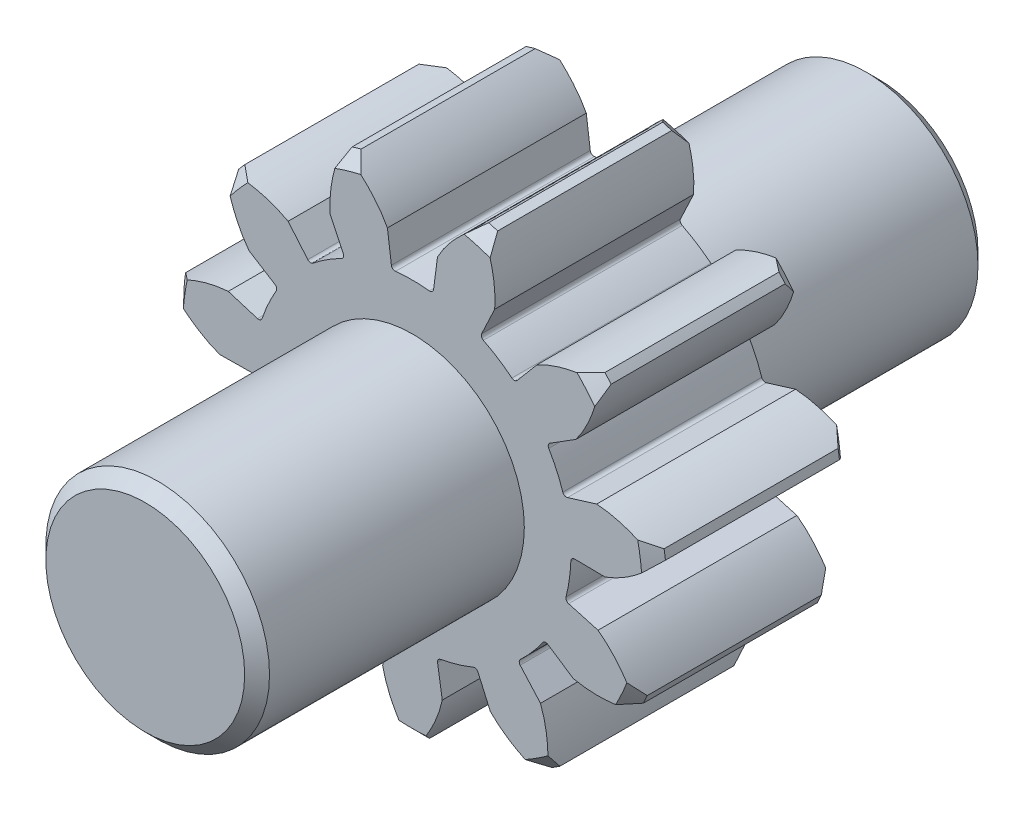
SolidWorks part; units mm, degrees
ref_plane "Middle plane" through (0, 0, 0) normal (0, 0, 1) x (1, 0, 0)
ref_plane "Top Plane" through (0, 0, 0) normal (0, 1, 0) x (1, 0, 0)
ref_plane "Right Plane" through (0, 0, 0) normal (1, 0, 0) x (0, 0, -1)
sketch "Spur gear" plane through (0, 0, 0) normal (0, 0, 1) x (1, 0, 0)
  line L0 (0, 0) -> (-2.3482, 16.3321) construction
  line L2 (-2.0154, 15.3734) -> (0, 0)
  line L3 (0, 0) -> (0, 52) construction
  line L4 (2.3482, 16.3321) -> (0, 0) construction
  line L6 (0, 0) -> (2.0154, 15.3734)
  circle A0 centre (0, 0) radius 15.5049
  circle A1 centre (0, 0) radius 12.75
  arc A2 (2.3482, 16.3321) -> (-2.3482, 16.3321) centre (0, 0) ccw
  circle A3 centre (0, 0) radius 19.5
  spline S0 degree 4 poles (0.7936, 14.8906) (0.7924, 14.9201) (0.7881, 14.9788) (0.7725, 15.0958) (0.7289, 15.316) (0.6484, 15.6067) (0.4539, 16.1447) (0.0492, 16.9597) (-0.6377, 17.9757) (-1.7913, 19.243) (-3.3499, 20.5096) (-5.2443, 21.6406) (-7.4338, 22.5657) (-9.7197, 23.2127) (-12.0632, 23.5974) (-14.5507, 23.7418) (-17.633, 23.5986) (-21.2621, 22.9576) (-25.3266, 21.6048) (-29.5547, 19.4226) (-33.4233, 16.6565) (-36.4497, 13.8025) (-38.7654, 11.0977) (-40.5023, 8.6952) (-41.7738, 6.6932) (-43.2134, 4.102) (-44.4514, 1.4058) (-45.4859, -1.3736) (-46.4831, -4.7889) (-47.0485, -7.396) (-47.4104, -9.7431) (-47.6077, -11.655) (-47.6802, -12.5487) (-47.7381, -13.4181) (-47.7759, -14.2391) (-47.8017, -14.99) (-47.8125, -16.0362) (-47.809, -16.7047) (-47.7875, -17.792) (-47.7473, -18.6332) (-47.688, -19.6577) (-47.6107, -20.5673) (-47.515, -21.548) (-47.4014, -22.4756) (-47.3026, -23.2033) (-47.2309, -23.6656) (-47.1936, -23.9061) knots 0 0 0 0 0 0.001401 0.002802 0.005604 0.010661 0.015718 0.02996 0.048734 0.068727 0.096889 0.125051 0.153212 0.181374 0.209535 0.237696 0.271429 0.327752 0.384075 0.440398 0.496721 0.553044 0.581206 0.609367 0.637529 0.66569 0.722013 0.750174 0.778336 0.834659 0.84874 0.86282 0.869861 0.876901 0.890982 0.900036 0.909091 0.920455 0.931818 0.943182 0.954545 0.965909 0.977273 0.988636 1 1 1 1 1 construction
  spline S1 degree 4 poles (-2.0154, 15.3734) (-2.1011, 15.5352) (-2.3813, 16.0225) (-2.9403, 16.8122) (-3.9842, 17.9417) (-5.4871, 19.1443) (-7.3108, 20.2145) (-9.4159, 21.0852) (-11.6114, 21.6888) (-13.8601, 22.0406) (-16.2451, 22.1609) (-19.1981, 22.0014) (-22.6715, 21.3607) (-26.557, 20.0349) (-30.5934, 17.9129) (-34.281, 15.2339) (-37.1607, 12.4768) (-39.3605, 9.8678) (-41.0077, 7.5528) (-42.2118, 5.6248) (-43.5728, 3.1311) (-44.7397, 0.5381) (-45.711, -2.1331) (-46.642, -5.4134) (-47.1651, -7.9161) (-47.4949, -10.1682) (-47.6701, -12.0019) (-47.7331, -12.8589) (-47.7823, -13.6926) (-47.8127, -14.4797) (-47.8319, -15.1995) (-47.8347, -16.2022) (-47.8265, -16.8429) (-47.798, -17.8848) (-47.7547, -18.6666) (-47.709, -19.3683) (-47.6743, -19.799) (-47.6569, -19.9982) knots 0.020881 0.020881 0.020881 0.020881 0.020881 0.02996 0.048734 0.068727 0.096889 0.125051 0.153212 0.181374 0.209535 0.237696 0.271429 0.327752 0.384075 0.440398 0.496721 0.553044 0.581206 0.609367 0.637529 0.66569 0.722013 0.750174 0.778336 0.834659 0.84874 0.86282 0.869861 0.876901 0.890982 0.900036 0.909091 0.920455 0.931818 0.943182 0.953189 0.953189 0.953189 0.953189 0.953189
  spline S2 degree 4 poles (-0.7936, 14.8906) (-0.7924, 14.9201) (-0.7881, 14.9788) (-0.7725, 15.0958) (-0.7289, 15.316) (-0.6484, 15.6067) (-0.4539, 16.1447) (-0.0492, 16.9597) (0.6377, 17.9757) (1.7913, 19.243) (3.3499, 20.5096) (5.2443, 21.6406) (7.4338, 22.5657) (9.7197, 23.2127) (12.0632, 23.5974) (14.5507, 23.7418) (17.633, 23.5986) (21.2621, 22.9576) (25.3266, 21.6048) (29.5547, 19.4226) (33.4233, 16.6565) (36.4497, 13.8025) (38.7654, 11.0977) (40.5023, 8.6952) (41.7738, 6.6932) (43.2134, 4.102) (44.4514, 1.4058) (45.4859, -1.3736) (46.4831, -4.7889) (47.0485, -7.396) (47.4104, -9.7431) (47.6077, -11.655) (47.6802, -12.5487) (47.7381, -13.4181) (47.7759, -14.2391) (47.8017, -14.99) (47.8125, -16.0362) (47.809, -16.7047) (47.7875, -17.792) (47.7473, -18.6332) (47.688, -19.6577) (47.6107, -20.5673) (47.515, -21.548) (47.4014, -22.4756) (47.3026, -23.2033) (47.2309, -23.6656) (47.1936, -23.9061) knots 0 0 0 0 0 0.001401 0.002802 0.005604 0.010661 0.015718 0.02996 0.048734 0.068727 0.096889 0.125051 0.153212 0.181374 0.209535 0.237696 0.271429 0.327752 0.384075 0.440398 0.496721 0.553044 0.581206 0.609367 0.637529 0.66569 0.722013 0.750174 0.778336 0.834659 0.84874 0.86282 0.869861 0.876901 0.890982 0.900036 0.909091 0.920455 0.931818 0.943182 0.954545 0.965909 0.977273 0.988636 1 1 1 1 1 construction
  spline S3 degree 4 poles (2.0154, 15.3734) (2.1011, 15.5352) (2.3813, 16.0225) (2.9403, 16.8122) (3.9842, 17.9417) (5.4871, 19.1443) (7.3108, 20.2145) (9.4159, 21.0852) (11.6114, 21.6888) (13.8601, 22.0406) (16.2451, 22.1609) (19.1981, 22.0014) (22.6715, 21.3607) (26.557, 20.0349) (30.5934, 17.9129) (34.281, 15.2339) (37.1607, 12.4768) (39.3605, 9.8678) (41.0077, 7.5528) (42.2118, 5.6248) (43.5728, 3.1311) (44.7397, 0.5381) (45.711, -2.1331) (46.642, -5.4134) (47.1651, -7.9161) (47.4949, -10.1682) (47.6701, -12.0019) (47.7331, -12.8589) (47.7823, -13.6926) (47.8127, -14.4797) (47.8319, -15.1995) (47.8347, -16.2022) (47.8265, -16.8429) (47.798, -17.8848) (47.7547, -18.6666) (47.709, -19.3683) (47.6743, -19.799) (47.6569, -19.9982) knots 0.020881 0.020881 0.020881 0.020881 0.020881 0.02996 0.048734 0.068727 0.096889 0.125051 0.153212 0.181374 0.209535 0.237696 0.271429 0.327752 0.384075 0.440398 0.496721 0.553044 0.581206 0.609367 0.637529 0.66569 0.722013 0.750174 0.778336 0.834659 0.84874 0.86282 0.869861 0.876901 0.890982 0.900036 0.909091 0.920455 0.931818 0.943182 0.953189 0.953189 0.953189 0.953189 0.953189
sketch "Circle" plane through (0, 0, 0) normal (0, 0, 1) x (1, 0, 0)
  circle A0 centre (0, 0) radius 19.5 construction
  circle A1 centre (0, 0) radius 19.5
extrude "Blank" add sketch "Circle" along normal mid plane 16
chamfer "Tooth chamfer" distance 1 angle 45 2 edges at (19.5, 0, -8) (19.5, 0, 8)
sketch "Tooth profile" plane through (0, 0, 0) normal (0, 0, 1) x (1, 0, 0)
  line L4 (0, 0) -> (2.0154, 15.3734) construction
  line L5 (-2.0154, 15.3734) -> (0, 0) construction
  line L6 (0, 0) -> (2.0154, 15.3734)
  line L7 (-2.0154, 15.3734) -> (0, 0)
  circle A4 centre (0, 0) radius 12.75 construction
  circle A5 centre (0, 0) radius 19.5 construction
  circle A6 centre (0, 0) radius 12.75
  circle A7 centre (0, 0) radius 19.5
  spline S1 degree 4 poles (999.7609, -51.6744) (36.065, -17.0379) (-0.5755, 0.4417) (-1.8205, 11.6607) (3.9842, 17.9417) (5.4871, 19.1443) (7.3108, 20.2145) (9.4159, 21.0852) (11.6114, 21.6888) (13.8601, 22.0406) (16.2451, 22.1609) (19.1981, 22.0014) (22.6715, 21.3607) (26.557, 20.0349) (30.5934, 17.9129) (34.281, 15.2339) (37.1607, 12.4768) (39.3605, 9.8678) (41.0077, 7.5528) (42.2118, 5.6248) (43.5728, 3.1311) (44.7397, 0.5381) (45.711, -2.1331) (46.642, -5.4134) (47.1651, -7.9161) (47.4949, -10.1682) (47.6701, -12.0019) (47.7331, -12.8589) (47.7823, -13.6926) (47.8127, -14.4797) (47.8319, -15.1995) (47.8347, -16.2022) (47.8265, -16.8429) (47.798, -17.8848) (47.5897, -21.6461) (46.8818, -29.7714) (46.3891, 13.6269) (33.8189, -1019.6941) knots -0.325788 -0.325788 -0.325788 -0.325788 -0.325788 0.02996 0.048734 0.068727 0.096889 0.125051 0.153212 0.181374 0.209535 0.237696 0.271429 0.327752 0.384075 0.440398 0.496721 0.553044 0.581206 0.609367 0.637529 0.66569 0.722013 0.750174 0.778336 0.834659 0.84874 0.86282 0.869861 0.876901 0.890982 0.900036 0.909091 0.920455 0.931818 0.943182 1.121242 1.121242 1.121242 1.121242 1.121242 only from (2.0154, 15.3734) to (47.6569, -19.9982) construction
  spline S3 degree 4 poles (-999.7609, -51.6744) (-36.065, -17.0379) (0.5755, 0.4417) (1.8205, 11.6607) (-3.9842, 17.9417) (-5.4871, 19.1443) (-7.3108, 20.2145) (-9.4159, 21.0852) (-11.6114, 21.6888) (-13.8601, 22.0406) (-16.2451, 22.1609) (-19.1981, 22.0014) (-22.6715, 21.3607) (-26.557, 20.0349) (-30.5934, 17.9129) (-34.281, 15.2339) (-37.1607, 12.4768) (-39.3605, 9.8678) (-41.0077, 7.5528) (-42.2118, 5.6248) (-43.5728, 3.1311) (-44.7397, 0.5381) (-45.711, -2.1331) (-46.642, -5.4134) (-47.1651, -7.9161) (-47.4949, -10.1682) (-47.6701, -12.0019) (-47.7331, -12.8589) (-47.7823, -13.6926) (-47.8127, -14.4797) (-47.8319, -15.1995) (-47.8347, -16.2022) (-47.8265, -16.8429) (-47.798, -17.8848) (-47.5897, -21.6461) (-46.8818, -29.7714) (-46.3891, 13.6269) (-33.8189, -1019.6941) knots -0.325788 -0.325788 -0.325788 -0.325788 -0.325788 0.02996 0.048734 0.068727 0.096889 0.125051 0.153212 0.181374 0.209535 0.237696 0.271429 0.327752 0.384075 0.440398 0.496721 0.553044 0.581206 0.609367 0.637529 0.66569 0.722013 0.750174 0.778336 0.834659 0.84874 0.86282 0.869861 0.876901 0.890982 0.900036 0.909091 0.920455 0.931818 0.943182 1.121242 1.121242 1.121242 1.121242 1.121242 only from (-2.0154, 15.3734) to (-47.6569, -19.9982) construction
  spline S4 degree 4 poles (2.0154, 15.3734) (2.1011, 15.5352) (2.3813, 16.0225) (2.9403, 16.8122) (3.9842, 17.9417) (5.4871, 19.1443) (7.3108, 20.2145) (9.4159, 21.0852) (11.6114, 21.6888) (13.8601, 22.0406) (16.2451, 22.1609) (19.1981, 22.0014) (22.6715, 21.3607) (26.557, 20.0349) (30.5934, 17.9129) (34.281, 15.2339) (37.1607, 12.4768) (39.3605, 9.8678) (41.0077, 7.5528) (42.2118, 5.6248) (43.5728, 3.1311) (44.7397, 0.5381) (45.711, -2.1331) (46.642, -5.4134) (47.1651, -7.9161) (47.4949, -10.1682) (47.6701, -12.0019) (47.7331, -12.8589) (47.7823, -13.6926) (47.8127, -14.4797) (47.8319, -15.1995) (47.8347, -16.2022) (47.8265, -16.8429) (47.798, -17.8848) (47.7547, -18.6666) (47.709, -19.3683) (47.6743, -19.799) (47.6569, -19.9982) knots 0.020881 0.020881 0.020881 0.020881 0.020881 0.02996 0.048734 0.068727 0.096889 0.125051 0.153212 0.181374 0.209535 0.237696 0.271429 0.327752 0.384075 0.440398 0.496721 0.553044 0.581206 0.609367 0.637529 0.66569 0.722013 0.750174 0.778336 0.834659 0.84874 0.86282 0.869861 0.876901 0.890982 0.900036 0.909091 0.920455 0.931818 0.943182 0.953189 0.953189 0.953189 0.953189 0.953189
  spline S5 degree 4 poles (-2.0154, 15.3734) (-2.1011, 15.5352) (-2.3813, 16.0225) (-2.9403, 16.8122) (-3.9842, 17.9417) (-5.4871, 19.1443) (-7.3108, 20.2145) (-9.4159, 21.0852) (-11.6114, 21.6888) (-13.8601, 22.0406) (-16.2451, 22.1609) (-19.1981, 22.0014) (-22.6715, 21.3607) (-26.557, 20.0349) (-30.5934, 17.9129) (-34.281, 15.2339) (-37.1607, 12.4768) (-39.3605, 9.8678) (-41.0077, 7.5528) (-42.2118, 5.6248) (-43.5728, 3.1311) (-44.7397, 0.5381) (-45.711, -2.1331) (-46.642, -5.4134) (-47.1651, -7.9161) (-47.4949, -10.1682) (-47.6701, -12.0019) (-47.7331, -12.8589) (-47.7823, -13.6926) (-47.8127, -14.4797) (-47.8319, -15.1995) (-47.8347, -16.2022) (-47.8265, -16.8429) (-47.798, -17.8848) (-47.7547, -18.6666) (-47.709, -19.3683) (-47.6743, -19.799) (-47.6569, -19.9982) knots 0.020881 0.020881 0.020881 0.020881 0.020881 0.02996 0.048734 0.068727 0.096889 0.125051 0.153212 0.181374 0.209535 0.237696 0.271429 0.327752 0.384075 0.440398 0.496721 0.553044 0.581206 0.609367 0.637529 0.66569 0.722013 0.750174 0.778336 0.834659 0.84874 0.86282 0.869861 0.876901 0.890982 0.900036 0.909091 0.920455 0.931818 0.943182 0.953189 0.953189 0.953189 0.953189 0.953189
extrude "Gear shaping" cut sketch "Tooth profile" against normal mid plane 16 contours S5 A6 S4 A7
fillet "Fillet1" [suppressed] radius 0.3
pattern_circular "CirPattern1" [suppressed] count 11 over 360
fillet "Fillet2" radius 0.3 2 edges at (1.6573, 12.6418, 0) (-1.6573, 12.6418, 0)
pattern_circular "CirPattern2" count 11 over 360 about axis through (0, 0, 8) along (0, 0, -1) of "Fillet2", "Gear shaping"
sketch "Pitch circle" plane through (0, 0, 0) normal (0, 0, 1) x (1, 0, 0)
  circle A0 centre (0, 0) radius 16.5 construction
  circle A1 centre (0, 0) radius 16.5 construction
sketch "Sketch2" plane through (0, 0, 8) normal (0, 0, 1) x (1, 0, 0)
  circle A0 centre (0, 0) radius 9
  dimension "D1" = 18
extrude "Boss-Extrude1" add sketch "Sketch2" along normal blind 21.5
sketch "Sketch3" plane through (0, 0, 29.5) normal (0, 0, 1) x (1, 0, 0)
  circle A0 centre (0, 0) radius 9
  dimension "D1" = 18
extrude "Boss-Extrude2" add sketch "Sketch3" against normal blind 59
chamfer "Chamfer1" distance 1 angle 45 2 edges at (9, 0, -29.5) (9, 0, 29.5)
equation "\"m\"= 3mm'模数"
equation "\"z\"= 11'齿数"
equation "\"a\"= 20'压力角（常见为20°）"
equation "\"B\"= 16'齿宽"
equation "\"C1\"= 1'轮齿倒角（若设为0，则无倒角）"
equation "\"x\"= 0'变位系数（不懂勿动）"
equation "\"ha\"= 1'齿顶高系数（不懂勿动）"
equation "\"c\"= 0.25'顶隙系数（不懂勿动）"
equation "\"基圆直径@Spur gear\"= \"m\" * \"z\" * cos ( \"a\" )"
equation "\"齿根圆@Spur gear\" = \"m\" * ( \"z\" - 2 * ( \"ha\" - \"x\" + \"c\" ) )"
equation "\"分度圆@Spur gear\"=\"m\" * \"z\""
equation "\"齿顶圆@Spur gear\" = \"m\" * ( \"z\" + 2 * ( \"ha\" + \"x\" ) )"
equation "\"R\"= 0.3'齿根圆角"
equation "\"D1\"= \"R\""
equation "\"D1@Blank\" = \"B\""
equation "\"D1@Tooth chamfer\" = IIF ( \"C1\" > 0 , \"C1\" , 0.001 )"
equation "\"轮齿倒角\"= IIF ( \"C1\" > 0 , \"unsuppressed\" , \"suppressed\" )"
equation "\"D1@Gear shaping\" = \"B\""
equation "\"D1@CirPattern1\" = \"z\""
equation "\"D1@Spur gear\"= \"m\" * ( pi / 2 ) - 2 * \"m\" * tan ( \"a\" ) * \"x\"'作者：机械菌-"
equation "\"D1@Fillet1\"=\"R\""
equation "\"圆角1\" = IIF ( \"m\" * ( \"z\" - 2 * ( \"ha\" - \"x\" + \"c\" ) ) > \"m\" * \"z\" * cos ( \"a\" ) , \"unsuppressed\" , \"suppressed\" )"
equation "\"圆周阵列1\"= IIF ( \"m\" * ( \"z\" - 2 * ( \"ha\" - \"x\" + \"c\" ) ) > \"m\" * \"z\" * cos ( \"a\" ) , \"unsuppressed\" , \"suppressed\" )"
equation "\"D1@Fillet2\"=\"R\""
equation "\"D1@CirPattern2\" = \"z\""
equation "\"圆角2\" = IIF ( \"m\" * ( \"z\" - 2 * ( \"ha\" - \"x\" + \"c\" ) ) < \"m\" * \"z\" * cos ( \"a\" ) , \"unsuppressed\" , \"suppressed\" )"
equation "\"圆周阵列2\"= IIF ( \"m\" *  ( \"z\" - 2 *  ( \"ha\" - \"x\" + \"c\" )  )  < \"m\" * \"z\" * cos ( \"a\" )  ,  unsuppressed  ,  suppressed  ) "
